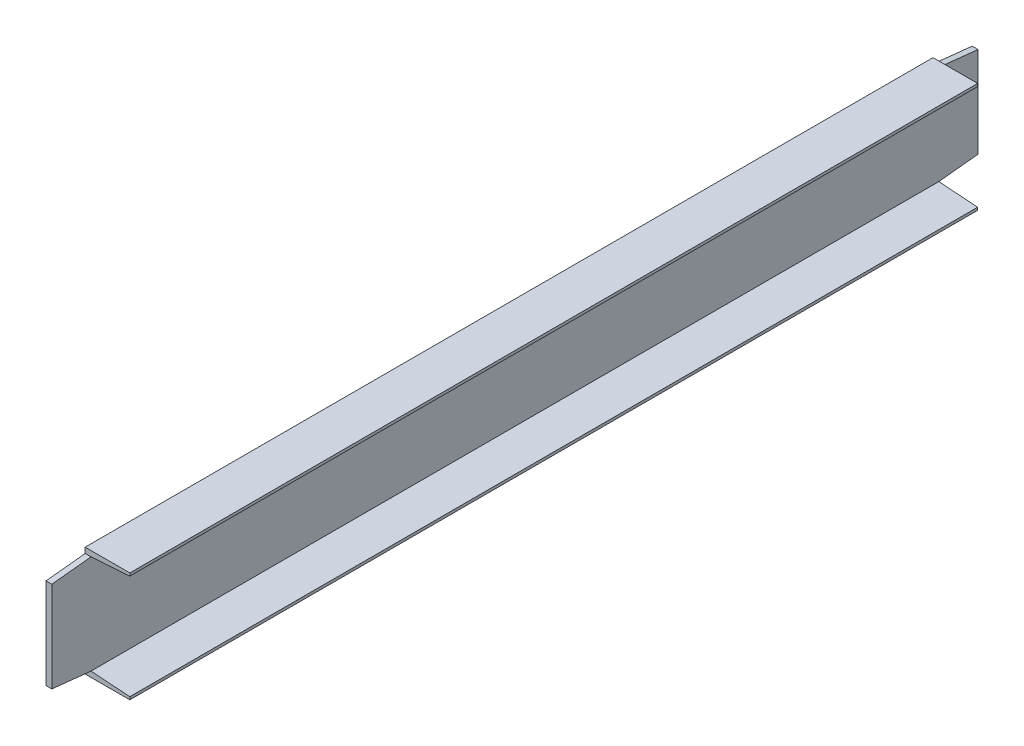
SolidWorks part; units mm, degrees
ref_plane "前视基准面" through (0, 0, 0) normal (0, 0, 1) x (1, 0, 0)
ref_plane "上视基准面" through (0, 0, 0) normal (0, 1, 0) x (1, 0, 0)
ref_plane "右视基准面" through (0, 0, 0) normal (1, 0, 0) x (0, 0, -1)
sketch "草图1" plane through (0, 0, 0) normal (0, 0, 1) x (1, 0, 0)
  line L0 (0, 0) -> (65, 0)
  line L1 (0, 0) -> (0, 160)
  line L2 (65, 156) -> (8.5, 152)
  line L3 (65, 0) -> (65, 4)
  line L4 (65, 4) -> (8.5, 8)
  line L5 (8.5, 8) -> (8.5, 152)
  line L6 (0, 80) -> (8.5, 80) construction
  line L7 (65, 160) -> (65, 156)
  line L8 (0, 160) -> (65, 160)
  dimension "D1" = 160
  dimension "D2" = 65
  dimension "D3" = 4
  dimension "D4" = 8.5
  dimension "D5" = 144
extrude "凸台-拉伸1" add sketch "草图1" along normal mid plane 1348
sketch "草图4" plane through (0, 0, 0) normal (-1, 0, 0) x (0, 0, 1)
  line L0 (-674, 160) -> (-617, 160)
  line L1 (674, 160) -> (-674, 160) construction
  line L2 (-617, 160) -> (-617, 152)
  line L3 (-617, 152) -> (-674, 146)
  line L4 (-674, 160) -> (-674, 0) construction
  line L5 (-674, 146) -> (-674, 160)
  line L6 (0, 160) -> (0, 0) construction
  line L7 (0, 80) -> (90.5463, 80) construction
  line L8 (674, 146) -> (674, 160)
  line L9 (617, 152) -> (674, 146)
  line L10 (617, 160) -> (617, 152)
  line L11 (674, 160) -> (617, 160)
  line L12 (674, 0) -> (617, 0)
  line L13 (617, 0) -> (617, 8)
  line L14 (617, 8) -> (674, 14)
  line L15 (674, 14) -> (674, 0)
  line L16 (-674, 14) -> (-674, 0)
  line L17 (-617, 8) -> (-674, 14)
  line L18 (-617, 0) -> (-617, 8)
  line L19 (-674, 0) -> (-617, 0)
  line L20 (674, 152) -> (-674, 152) construction
  point P5 (-674, 80)
  dimension "D1" = 57
  dimension "D2" = 66
extrude "切除-拉伸1" cut sketch "草图4" against normal through all
